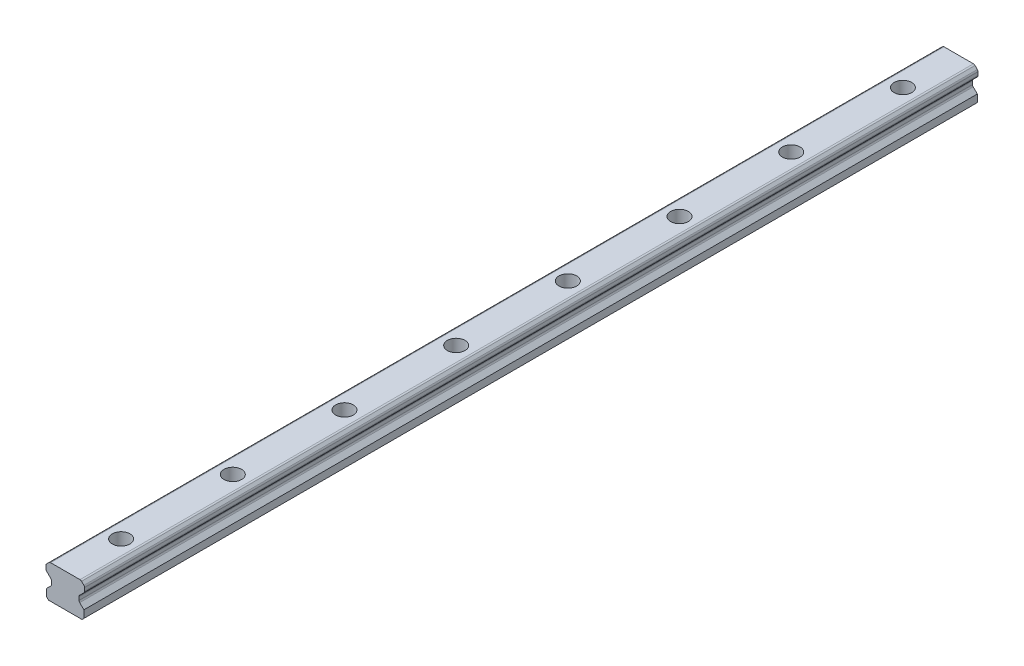
from build123d import *

# Parameters (mm, degrees)
BOSS_EXTRUDE1_DEPTH           = 480
COUNTERSINK_HOLE1_D           = 6
COUNTERSINK_HOLE1_CBORE_D     = 9.5
COUNTERSINK_HOLE1_CBORE_DEPTH = 8.5
LPATTERN1_COUNT               = 8
LPATTERN1_PITCH               = 60
CHAMFER1_SIZE                 = 1


with BuildPart() as part:
    # Sketch3 → Boss-Extrude1 (new body)
    with BuildSketch(Plane.XY):
        with BuildLine():
            Line((-10, -5), (10, -5))
            Line((10, -5), (10, 0))
            Line((10, 0), (7.7627417, 2.2372583))
            ThreePointArc((7.7627417, 2.2372583), (7.502614398, 2.626566319), (7.411269837, 3.085786438))
            Line((7.411269837, 3.085786438), (7.411269837, 4.851471863))
            ThreePointArc((7.411269837, 4.851471863), (7.502614398, 5.310691981), (7.7627417, 5.7))
            Line((7.7627417, 5.7), (10, 7.9372583))
            ThreePointArc((10, 7.9372583), (10.260127302, 8.326566319), (10.351471863, 8.785786438))
            Line((10.351471863, 8.785786438), (10.351471863, 10.551471863))
            ThreePointArc((10.351471863, 10.551471863), (10.260127302, 11.010691981), (10, 11.4))
            Line((10, 11.4), (8.751471863, 12.648528137))
            ThreePointArc((8.751471863, 12.648528137), (8.362163844, 12.908655439), (7.902943725, 13))
            Line((7.902943725, 13), (-7.902943725, 13))
            ThreePointArc((-7.902943725, 13), (-8.362163844, 12.908655439), (-8.751471863, 12.648528137))
            Line((-8.751471863, 12.648528137), (-10, 11.4))
            ThreePointArc((-10, 11.4), (-10.260127302, 11.010691981), (-10.351471863, 10.551471863))
            Line((-10.351471863, 10.551471863), (-10.351471863, 8.785786438))
            ThreePointArc((-10.351471863, 8.785786438), (-10.260127302, 8.326566319), (-10, 7.9372583))
            Line((-10, 7.9372583), (-7.7627417, 5.7))
            ThreePointArc((-7.7627417, 5.7), (-7.502614398, 5.310691981), (-7.411269837, 4.851471863))
            Line((-7.411269837, 4.851471863), (-7.411269837, 3.085786438))
            ThreePointArc((-7.411269837, 3.085786438), (-7.502614398, 2.626566319), (-7.7627417, 2.2372583))
            Line((-7.7627417, 2.2372583), (-10, 0))
            Line((-10, 0), (-10, -5))
        make_face()
    extrude(amount=-BOSS_EXTRUDE1_DEPTH)

    # Countersink Hole1 (through all)
    with Locations(Plane(origin=(0, 13, 0), x_dir=(-1, 0, 0), z_dir=(0, 1, 0))):
        with Locations((0, -30)):
            countersink_hole1 = CounterBoreHole(COUNTERSINK_HOLE1_D / 2, COUNTERSINK_HOLE1_CBORE_D / 2, COUNTERSINK_HOLE1_CBORE_DEPTH)

    # LPattern1: Countersink Hole1 ×8
    with Locations(*[(0, 0, -i * LPATTERN1_PITCH) for i in range(1, LPATTERN1_COUNT)]):
        add(countersink_hole1, mode=Mode.SUBTRACT)

    # Chamfer1
    chamfer1_edges = [part.edges().sort_by_distance(p)[0] for p in [
        (10, -5, -240),
        (-10, -5, -240),
    ]]
    chamfer(chamfer1_edges, length=CHAMFER1_SIZE)


solid = part.part
